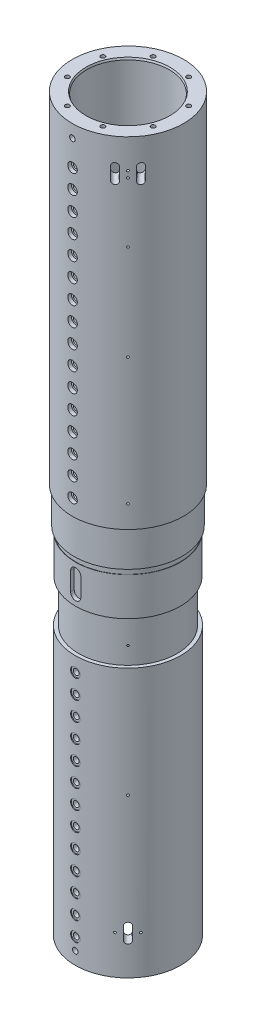
from build123d import *
from OCP.BRepFilletAPI import BRepFilletAPI_MakeChamfer

# Parameters (mm, degrees)
SKETCH1_R                = 87.5
SKETCH1_R_2              = 65
BOSS_EXTRUDE1_DEPTH      = 1149
CIRPATTERN1_COUNT        = 8
CUT_EXTRUDE13_REACH      = 1170.257
CUT_EXTRUDE13_END_RADIUS = 65
M4_TAPPED_HOLE2_D        = 3.3
M4_TAPPED_HOLE2_DEPTH    = 11.5
M4_TAPPED_HOLE2_TIP      = 0.991420021
CUT_EXTRUDE14_REACH      = 1170.257
CUT_EXTRUDE14_END_RADIUS = 65
M4_TAPPED_HOLE3_D        = 3.3
M4_TAPPED_HOLE3_DEPTH    = 11.5
M4_TAPPED_HOLE3_TIP      = 0.991420021
G1_8_TAPPED_HOLE1_D      = 8.8
G1_8_TAPPED_HOLE1_DEPTH  = 22.18
G1_8_TAPPED_HOLE1_TIP    = 2.643786724
M4_TAPPED_HOLE4_D        = 3.3
M4_TAPPED_HOLE4_DEPTH    = 11.5
M4_TAPPED_HOLE4_TIP      = 0.991420021
SKETCH47_R               = 141.946542251
SKETCH47_R_2             = 85
CUT_EXTRUDE19_DEPTH      = 614
CUT_EXTRUDE20_START      = 56
SKETCH48_R               = 100.445814599
SKETCH48_R_2             = 82
CUT_EXTRUDE20_DEPTH      = 9
SKETCH54_OUTSIDE_W       = 412.07
SKETCH54_OUTSIDE_H       = 412.07
SKETCH54_OUTSIDE_R       = 83
CUT_EXTRUDE26_DEPTH      = 550
SKETCH55_OUTSIDE_W       = 412.07
SKETCH55_OUTSIDE_H       = 412.07
SKETCH55_OUTSIDE_R       = 82.5
CUT_EXTRUDE27_DEPTH      = 69
SKETCH56_OUTSIDE_W       = 412.07
SKETCH56_OUTSIDE_H       = 412.07
SKETCH56_OUTSIDE_R       = 77.5
CUT_EXTRUDE28_DEPTH      = 67
SKETCH57_R               = 67.5
CUT_EXTRUDE29_DEPTH      = 14
CUT_EXTRUDE30_DEPTH      = 11
CIRPATTERN2_COUNT        = 8
LPATTERN1_COUNT          = 36
LPATTERN1_PITCH          = 30
CHAMFER1_SIZE            = 3
CHAMFER1_SIZE2           = 1.091910703
CHAMFER2_SIZE            = 2
CHAMFER2_SIZE2           = 0.727940469


with BuildPart() as part:
    # Sketch1 → Boss-Extrude1 (new body)
    with BuildSketch(Plane(origin=(0, 0, 0), x_dir=(1, 0, 0), z_dir=(0, 1, 0))):
        with Locations(Location((0, 0, 0), (0, 0, 270))):
            Circle(SKETCH1_R)
        with Locations(Location((0, 0, 0), (0, 0, 270))):
            Circle(SKETCH1_R_2, mode=Mode.SUBTRACT)
    extrude(amount=BOSS_EXTRUDE1_DEPTH)

    # Sketch19 → M8 Tapped Hole1 (revolve, cut)
    with BuildSketch(Plane(origin=(27.935890563, 1149, 67.443205873), x_dir=(0, 0, 1), z_dir=(1, 0, 0))):
        Polygon((0, 0), (0, 33.292926105), (3.4, 31.25), (3.4, 0), align=None)
    m8_tapped_hole1 = revolve(axis=Axis((27.935890563, 1155.35, 67.443205873), (0, -1, 0)), mode=Mode.SUBTRACT)

    # Sketch21 → M8 Tapped Hole2 (revolve, cut)
    with BuildSketch(Plane(origin=(27.935890563, 0, 67.443205873), x_dir=(0, 0, -1), z_dir=(1, 0, 0))):
        Polygon((0, 0), (0, 38.292926105), (3.4, 36.25), (3.4, 0), align=None)
    m8_tapped_hole2 = revolve(axis=Axis((27.935890563, -6.35, 67.443205873), (0, 1, 0)), mode=Mode.SUBTRACT)

    # CirPattern1: M8 Tapped Hole2 ×8 about axis
    cirpattern1_axis = Axis((0, 0, 0), (0, 1, 0))
    for i in range(1, CIRPATTERN1_COUNT):
        add(m8_tapped_hole2.rotate(cirpattern1_axis, i * 360 / CIRPATTERN1_COUNT), mode=Mode.SUBTRACT)

    # Sketch25 → Hole size (% based on socket head cap screw type)3 (revolve, cut)
    with BuildSketch(Plane(origin=(0, 1089, 87.5), x_dir=(0, -1, 0), z_dir=(1, 0, 0))):
        Polygon((0, 0), (0, 82.703872786), (4.5, 80), (4.5, 6), (7.5, 6), (7.5, 0), align=None)
    hole_size_based_on_socket_head_cap_scr = revolve(axis=Axis((0, 1089, 93.85), (0, 0, -1)), mode=Mode.SUBTRACT)

    # Cut-Extrude13: up to this cylinder (the profile starts outside it)
    cut_extrude13_end = Plane(origin=(0, 1098, 0), z_dir=(0, -1, 0)) * Cylinder(CUT_EXTRUDE13_END_RADIUS, 2471.514, mode=Mode.PRIVATE)
    # Sketch29 → Cut-Extrude13 (cut, up to the surface)
    with BuildSketch(Plane(origin=(61.871843354, 0, 61.871843354), x_dir=(0, -1, 0), z_dir=(0.7071067811865488, 0, 0.7071067811865464)), mode=Mode.PRIVATE) as cut_extrude13_sk1:
        with BuildLine():
            Line((-1108, 19.5), (-1088, 19.5))
            ThreePointArc((-1088, 19.5), (-1083, 14.5), (-1088, 9.5))
            Line((-1088, 9.5), (-1108, 9.5))
            ThreePointArc((-1108, 9.5), (-1113, 14.5), (-1108, 19.5))
        make_face()
    cut_extrude13_tool1 = extrude(cut_extrude13_sk1.sketch, amount=-CUT_EXTRUDE13_REACH, mode=Mode.PRIVATE) - cut_extrude13_end
    add(cut_extrude13_tool1.solids().sort_by_distance((72.124892, 1098, 51.618795))[0], mode=Mode.SUBTRACT)
    # Sketch29 → Cut-Extrude13 (cut, up to the surface)
    with BuildSketch(Plane(origin=(61.871843354, 0, 61.871843354), x_dir=(0, -1, 0), z_dir=(0.7071067811865488, 0, 0.7071067811865464)), mode=Mode.PRIVATE) as cut_extrude13_sk2:
        with BuildLine():
            Line((-1108, -9.5), (-1088, -9.5))
            ThreePointArc((-1088, -9.5), (-1083, -14.5), (-1088, -19.5))
            Line((-1088, -19.5), (-1108, -19.5))
            ThreePointArc((-1108, -19.5), (-1113, -14.5), (-1108, -9.5))
        make_face()
    cut_extrude13_tool2 = extrude(cut_extrude13_sk2.sketch, amount=-CUT_EXTRUDE13_REACH, mode=Mode.PRIVATE) - cut_extrude13_end
    add(cut_extrude13_tool2.solids().sort_by_distance((51.618795, 1098, 72.124892))[0], mode=Mode.SUBTRACT)

    # M4 Tapped Hole2
    with Locations(Plane(origin=(61.871843354, 0, 61.871843354), x_dir=(0, -1, 0), z_dir=(0.7071067811865488, 0, 0.7071067811865464))):
        with Locations((-1103, 0), (-1093, 0)):
            Hole(M4_TAPPED_HOLE2_D / 2, depth=M4_TAPPED_HOLE2_DEPTH)
            with Locations((0, 0, -(M4_TAPPED_HOLE2_DEPTH + M4_TAPPED_HOLE2_TIP / 2))):  # 118° drill point
                Cone(0, M4_TAPPED_HOLE2_D / 2, M4_TAPPED_HOLE2_TIP, mode=Mode.SUBTRACT)

    # Cut-Extrude14: up to this cylinder (the profile starts outside it)
    cut_extrude14_end = Plane(origin=(0, 61, 0), z_dir=(0, -1, 0)) * Cylinder(CUT_EXTRUDE14_END_RADIUS, 2471.514, mode=Mode.PRIVATE)
    # Sketch32 → Cut-Extrude14 (cut, up to the surface)
    with BuildSketch(Plane(origin=(61.871843354, 0, 61.871843354), x_dir=(0, -1, 0), z_dir=(0.7071067811865488, 0, 0.7071067811865464)), mode=Mode.PRIVATE) as cut_extrude14_sk1:
        with BuildLine():
            Line((-51, -5), (-71, -5))
            ThreePointArc((-71, -5), (-76, 0), (-71, 5))
            Line((-71, 5), (-51, 5))
            ThreePointArc((-51, 5), (-46, 0), (-51, -5))
        make_face()
    cut_extrude14_tool1 = extrude(cut_extrude14_sk1.sketch, amount=-CUT_EXTRUDE14_REACH, mode=Mode.PRIVATE) - cut_extrude14_end
    add(cut_extrude14_tool1.solids().sort_by_distance((61.871843, 61, 61.871843))[0], mode=Mode.SUBTRACT)

    # M4 Tapped Hole3
    with Locations(Plane(origin=(61.871843354, 0, 61.871843354), x_dir=(0, -1, 0), z_dir=(0.7071067811865488, 0, 0.7071067811865464))):
        with Locations((-61, 14.5), (-61, -14.5)):
            Hole(M4_TAPPED_HOLE3_D / 2, depth=M4_TAPPED_HOLE3_DEPTH)
            with Locations((0, 0, -(M4_TAPPED_HOLE3_DEPTH + M4_TAPPED_HOLE3_TIP / 2))):  # 118° drill point
                Cone(0, M4_TAPPED_HOLE3_D / 2, M4_TAPPED_HOLE3_TIP, mode=Mode.SUBTRACT)

    # G1/8 Tapped Hole1
    with Locations(Plane.XY.offset(87.5)):
        with Locations((0, 20), (0, 1129)):
            Hole(G1_8_TAPPED_HOLE1_D / 2, depth=G1_8_TAPPED_HOLE1_DEPTH)
            with Locations((0, 0, -(G1_8_TAPPED_HOLE1_DEPTH + G1_8_TAPPED_HOLE1_TIP / 2))):  # 118° drill point
                Cone(0, G1_8_TAPPED_HOLE1_D / 2, G1_8_TAPPED_HOLE1_TIP, mode=Mode.SUBTRACT)

    # M4 Tapped Hole4
    with Locations(Plane(origin=(61.871843354, 0, 61.871843354), x_dir=(0, -1, 0), z_dir=(0.7071067811865488, 0, 0.7071067811865464))):
        with Locations((-999, 0), (-849, 0), (-649, 0), (-449, 0), (-249, 0)):
            Hole(M4_TAPPED_HOLE4_D / 2, depth=M4_TAPPED_HOLE4_DEPTH)
            with Locations((0, 0, -(M4_TAPPED_HOLE4_DEPTH + M4_TAPPED_HOLE4_TIP / 2))):  # 118° drill point
                Cone(0, M4_TAPPED_HOLE4_D / 2, M4_TAPPED_HOLE4_TIP, mode=Mode.SUBTRACT)

    # Sketch47 → Cut-Extrude19 (cut)
    with BuildSketch(Plane(origin=(0, 0, 0), x_dir=(1, 0, 0), z_dir=(0, 1, 0))):
        Circle(SKETCH47_R)
        with Locations(Location((0, 0, 0), (0, 0, 270))):
            Circle(SKETCH47_R_2, mode=Mode.SUBTRACT)
    extrude(amount=CUT_EXTRUDE19_DEPTH, mode=Mode.SUBTRACT)

    # Sketch48 → Cut-Extrude20 (cut)
    with BuildSketch(Plane.XZ.offset(-614).offset(CUT_EXTRUDE20_START)):
        Circle(SKETCH48_R)
        with Locations(Location((0, 0, 0), (0, 0, 270))):
            Circle(SKETCH48_R_2, mode=Mode.SUBTRACT)
    extrude(amount=CUT_EXTRUDE20_DEPTH, mode=Mode.SUBTRACT)

    # Sketch54 outside → Cut-Extrude26 (cut)
    with BuildSketch(Plane.XZ):
        Rectangle(SKETCH54_OUTSIDE_W, SKETCH54_OUTSIDE_H)
        with Locations(Location((0, 0, 0), (0, 0, 270))):
            Circle(SKETCH54_OUTSIDE_R, mode=Mode.SUBTRACT)
    extrude(amount=-CUT_EXTRUDE26_DEPTH, mode=Mode.SUBTRACT)

    # Sketch55 outside → Cut-Extrude27 (cut)
    with BuildSketch(Plane.XZ.offset(-558)):
        Rectangle(SKETCH55_OUTSIDE_W, SKETCH55_OUTSIDE_H)
        with Locations(Location((0, 0, 0), (0, 0, 270))):
            Circle(SKETCH55_OUTSIDE_R, mode=Mode.SUBTRACT)
    extrude(amount=CUT_EXTRUDE27_DEPTH, mode=Mode.SUBTRACT)

    # Sketch56 outside → Cut-Extrude28 (cut)
    with BuildSketch(Plane(origin=(0, 489, 0), x_dir=(1, 0, 0), z_dir=(0, 1, 0))):
        Rectangle(SKETCH56_OUTSIDE_W, SKETCH56_OUTSIDE_H)
        with Locations(Location((0, 0, 0), (0, 0, 270))):
            Circle(SKETCH56_OUTSIDE_R, mode=Mode.SUBTRACT)
    extrude(amount=-CUT_EXTRUDE28_DEPTH, mode=Mode.SUBTRACT)

    # Sketch57 → Cut-Extrude29 (cut)
    with BuildSketch(Plane.XZ):
        with Locations(Location((0, 0, 0), (0, 0, 270))):
            Circle(SKETCH57_R)
    extrude(amount=-CUT_EXTRUDE29_DEPTH, mode=Mode.SUBTRACT)

    # Sketch58 → Cut-Extrude30 (cut)
    with BuildSketch(Plane.XY.offset(87.5)):
        with BuildLine():
            Line((-8, 504.5), (-8, 533.5))
            ThreePointArc((-8, 533.5), (0, 541.5), (8, 533.5))
            Line((8, 533.5), (8, 504.5))
            ThreePointArc((8, 504.5), (0, 496.5), (-8, 504.5))
        make_face()
    extrude(amount=-CUT_EXTRUDE30_DEPTH, mode=Mode.SUBTRACT)

    # CirPattern2: M8 Tapped Hole1 ×8 about axis
    cirpattern2_axis = Axis((0, 0, 0), (0, 1, 0))
    for i in range(1, CIRPATTERN2_COUNT):
        add(m8_tapped_hole1.rotate(cirpattern2_axis, i * 360 / CIRPATTERN2_COUNT), mode=Mode.SUBTRACT)

    # LPattern1: Hole size (% based on socket head cap screw type)3 ×36, 7 skipped
    with Locations(*[(0, -i * LPATTERN1_PITCH, 0) for i in range(1, LPATTERN1_COUNT) if i not in (16, 17, 18, 19, 20, 21, 22)]):
        add(hole_size_based_on_socket_head_cap_scr, mode=Mode.SUBTRACT)

    # Chamfer1: one chamfer whose edges measure the first distance from different faces: ONE call of the kernel's chamfer builder (chamfer() names one face for all edges)
    chamfer1_edges_1 = [part.edges().sort_by_distance(p)[0] for p in [
        (0, 0, 67.5),
    ]]
    chamfer1_side_1 = [part.faces().sort_by_distance(p)[0] for p in [
        (0, 7, 67.5),
    ]]
    chamfer1_edges_2 = [part.edges().sort_by_distance(p)[0] for p in [
        (0, 1149, -65),
    ]]
    chamfer1_side_2 = [part.faces().sort_by_distance(p)[0] for p in [
        (0, 581.5, -65),
    ]]
    chamfer1 = BRepFilletAPI_MakeChamfer(part.part.solid().wrapped)
    for e in chamfer1_edges_1:
        chamfer1.Add(CHAMFER1_SIZE, CHAMFER1_SIZE2, e.wrapped, chamfer1_side_1[0].wrapped)  # the first distance lies on this face
    for e in chamfer1_edges_2:
        chamfer1.Add(CHAMFER1_SIZE, CHAMFER1_SIZE2, e.wrapped, chamfer1_side_2[0].wrapped)  # the first distance lies on this face
    add(Compound.cast(chamfer1.Shape()), mode=Mode.REPLACE)

    # Chamfer2
    chamfer2_edges = [part.edges().sort_by_distance(p)[0] for p in [
        (0, 14, -65),
    ]]
    chamfer2_side = [part.faces().sort_by_distance(p)[0] for p in [
        (0, 580, -65),
    ]]
    chamfer(chamfer2_edges, length=CHAMFER2_SIZE, length2=CHAMFER2_SIZE2, reference=chamfer2_side[0])


solid = part.part
